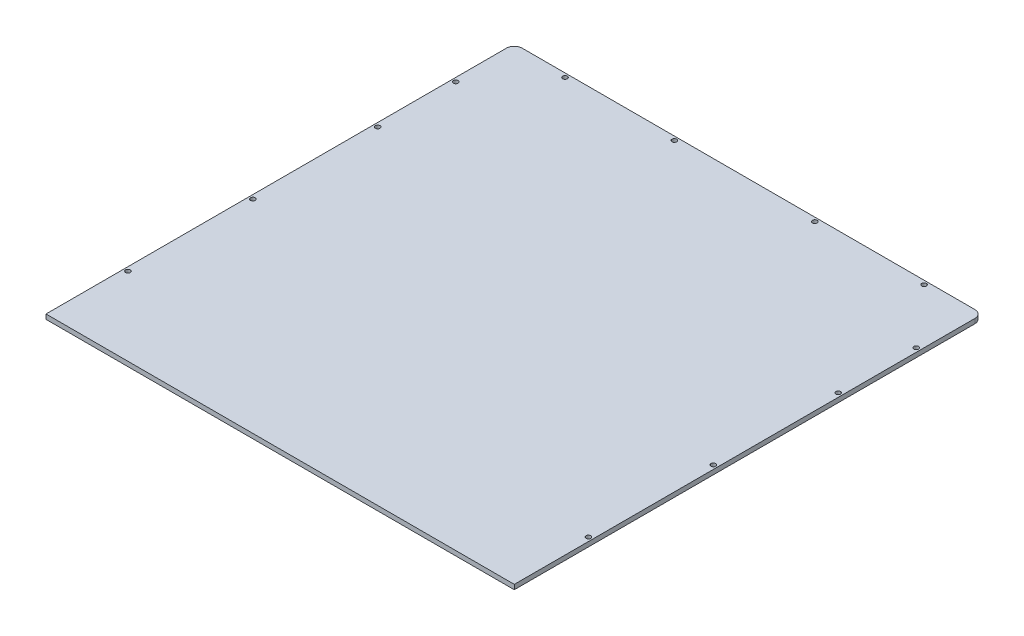
from build123d import *

# Parameters (mm, degrees)
SKETCH1_R           = 1.5
BOSS_EXTRUDE1_DEPTH = 3


with BuildPart() as part:
    # Sketch1 → Boss-Extrude1 (new body)
    with BuildSketch(Plane(origin=(0, 0, 0), x_dir=(1, 0, 0), z_dir=(0, 1, 0))):
        with BuildLine():
            Line((-150, -150), (150, -150))
            Line((150, -150), (150, 145))
            ThreePointArc((150, 145), (148.535533906, 148.535533906), (145, 150))
            Line((145, 150), (-145, 150))
            ThreePointArc((-145, 150), (-148.535533906, 148.535533906), (-150, 145))
            Line((-150, 145), (-150, -150))
        make_face()
        with Locations(Location((-147.5, -100, 0), (0, 0, 270))):
            Circle(SKETCH1_R, mode=Mode.SUBTRACT)
        with Locations(Location((-147.5, -20, 0), (0, 0, 270))):
            Circle(SKETCH1_R, mode=Mode.SUBTRACT)
        with Locations(Location((-147.5, 60, 0), (0, 0, 270))):
            Circle(SKETCH1_R, mode=Mode.SUBTRACT)
        with Locations(Location((-147.5, 110, 0), (0, 0, 270))):
            Circle(SKETCH1_R, mode=Mode.SUBTRACT)
        with Locations(Location((-115, 147.5, 0), (0, 0, 270))):
            Circle(SKETCH1_R, mode=Mode.SUBTRACT)
        with Locations(Location((-45, 147.5, 0), (0, 0, 270))):
            Circle(SKETCH1_R, mode=Mode.SUBTRACT)
        with Locations(Location((45, 147.5, 0), (0, 0, 90))):
            Circle(SKETCH1_R, mode=Mode.SUBTRACT)
        with Locations(Location((115, 147.5, 0), (0, 0, 90))):
            Circle(SKETCH1_R, mode=Mode.SUBTRACT)
        with Locations(Location((147.5, -20, 0), (0, 0, 90))):
            Circle(SKETCH1_R, mode=Mode.SUBTRACT)
        with Locations(Location((147.5, -100, 0), (0, 0, 90))):
            Circle(SKETCH1_R, mode=Mode.SUBTRACT)
        with Locations(Location((147.5, 110, 0), (0, 0, 90))):
            Circle(SKETCH1_R, mode=Mode.SUBTRACT)
        with Locations(Location((147.5, 60, 0), (0, 0, 90))):
            Circle(SKETCH1_R, mode=Mode.SUBTRACT)
    extrude(amount=BOSS_EXTRUDE1_DEPTH)


solid = part.part
